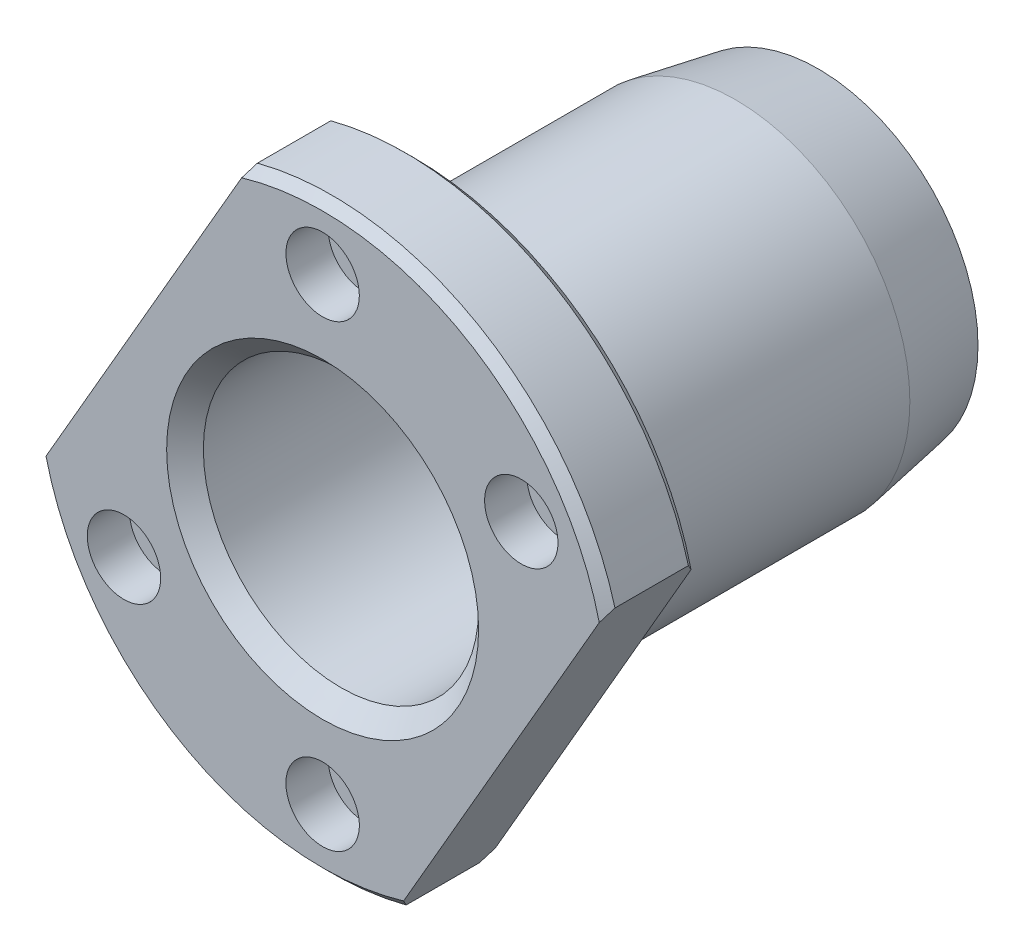
SolidWorks part; units mm, degrees
material "Nylon 66"
ref_plane "Front Plane" through (0, 0, 0) normal (0, 0, 1) x (1, 0, 0)
ref_plane "Top Plane" through (0, 0, 0) normal (0, 1, 0) x (1, 0, 0)
ref_plane "Right Plane" through (0, 0, 0) normal (1, 0, 0) x (0, 0, -1)
sketch "Sketch1" plane through (0, 0, 0) normal (0, 0, 1) x (1, 0, 0)
  circle A0 centre (0, 0) radius 19
  dimension "D1" = 38
extrude "Boss-Extrude1" add sketch "Sketch1" along normal blind 45
sketch "Sketch2" plane through (0, 0, 45) normal (0, 0, 1) x (1, 0, 0)
  circle A0 centre (0, 0) radius 15
  dimension "D1" = 30
extrude "Cut-Extrude1" cut sketch "Sketch2" against normal offset from surface (30 mm away) 15 up to face at (19, 0, 0)
hole_wizard "M18x1.5 Tapped Hole1" positions "3DSketch1" profile "Sketch4" tap size "M18x1.5" standard "Gb"
sketch3d "3DSketch1"
  point P0 (0, 0, 0)
sketch "Sketch4" plane through (0, 0, 0) normal (1, 0, 0) x (0, 1, 0)
  line L0 (0, 0) -> (0, 48.4571)
  line L1 (0, 48.4571) -> (8.25, 43.5)
  line L2 (8.25, 43.5) -> (8.25, 0)
  line L5 (8.25, 0) -> (0, 0)
  line L10 (0, 48.4571) -> (-8.25, 43.5) construction
  line L11 (0, -6.35) -> (0, 107.95) construction
  dimension "螺纹孔钻头直径" = 16.5
  dimension "螺纹孔钻头深度" = 43.5
  dimension "导头角度" = 118
cosmetic thread "Cosmetic Thread1" parameters "D1"=15, "D2"=18
sketch "Sketch5" plane through (0, 0, 45) normal (0, 0, 1) x (1, 0, 0)
  circle A0 centre (0, 0) radius 32
  circle A2 centre (0, 0) radius 15 construction
  circle A3 centre (0, 0) radius 15
  dimension "D1" = 64
extrude "Boss-Extrude2" add sketch "Sketch5" along normal blind 10
hole_wizard "Hole size per socket head cap screw type1" positions "3DSketch2" profile "Sketch6" counterbore size "M4" standard "Gb" end condition through all
sketch3d "3DSketch2"
  line L0 (0, 25, 55) -> (0, 0, 55) construction
  line L1 (0, 0, 15) -> (0, 0, 55) construction
  line L2 (0, 0, 55) -> (0, 0, 45) construction
  point P0 (0, 25, 55)
  dimension "D1" = 25
sketch "Sketch6" plane through (0, 25, 55) normal (1, 0, 0) x (0, -1, 0)
  line L0 (0, 0) -> (0, 55)
  line L1 (0, 55) -> (2.25, 55)
  line L3 (2.25, 55) -> (2.25, 4.6)
  line L4 (2.25, 4.6) -> (4, 4.6)
  line L5 (4, 4.6) -> (4, 0)
  line L7 (4, 0) -> (0, 0)
  line L11 (0, -6.35) -> (0, 107.95) construction
  dimension "通孔孔直径" = 4.5
  dimension "通孔孔深度" = 55
  dimension "柱形沉头孔直径" = 8
  dimension "柱形沉头孔深度" = 4.6
pattern_circular "CirPattern1" count 6 over 360 about axis through (0, 0, 55) along (0, 0, 1) skipping 1, 4 of "Hole size per socket head cap screw type1"
sketch "Sketch7" plane through (0, 0, 55) normal (0, 0, 1) x (1, 0, 0)
  line L0 (0, 25) -> (-21.6506, -12.5) construction
  line L1 (21.6506, 12.5) -> (0, -25) construction
  line L2 (-8.1085, 30.9556) -> (-30.8626, -8.4556)
  line L3 (30.8626, 8.4556) -> (8.1085, -30.9556)
  line L4 (-8.6603, 30) -> (-30.3109, -7.5) construction
  line L5 (30.3109, 7.5) -> (8.6603, -30) construction
  circle A1 centre (0, 0) radius 32 construction
  arc A2 (-8.1085, 30.9556) -> (-30.8626, -8.4556) centre (0, 0) ccw
  arc A3 (8.1085, -30.9556) -> (30.8626, 8.4556) centre (0, 0) ccw
  dimension "D1" = 10
  dimension "D2" = 10
extrude "Cut-Extrude2" cut sketch "Sketch7" against normal up to next
chamfer "Chamfer1" distance 1 angle 45 4 edges at (16, 27.7128, 45) (-16, -27.7128, 45) (16, 27.7128, 55) (-16, -27.7128, 55)
chamfer "Chamfer2" distance 10 angle 10 1 edges at (19, 0, 0)
chamfer "Chamfer3" distance 1 angle 45 1 edges at (17.2367, 0, 0)
chamfer "Chamfer4" distance 2 angle 45 1 edges at (15, 0, 55)
